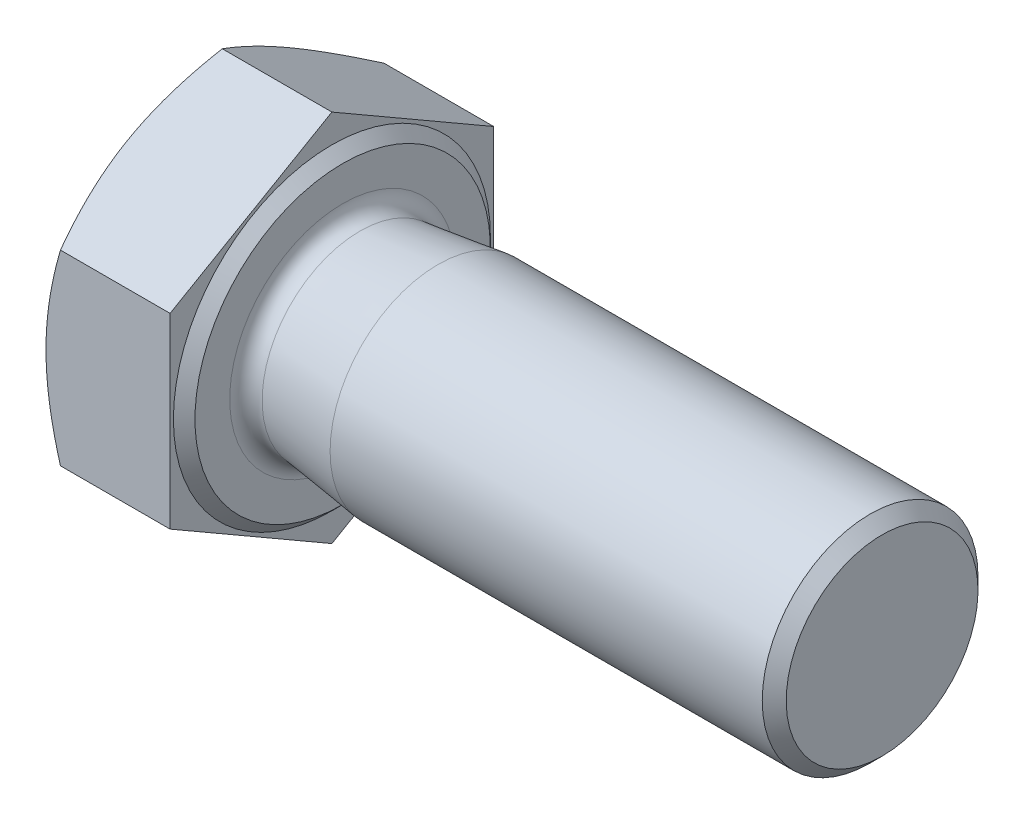
from build123d import *

# Parameters (mm, degrees)
EXTRUDE_1_DEPTH     = 7.5
SKETCH_4_R          = 20.03
SKETCH_4_R_2        = 9
CUT_EXTRUDE_1_DEPTH = 0.9375
CUT_EXTRUDE_1_DRAFT = -60
CHAMFER_1_SIZE      = 0.666666667


with BuildPart() as part:
    # 草图3 → 凸台-拉伸1 (new body)
    with BuildSketch(Plane(origin=(0, 0, 0), x_dir=(0, 0, -1), z_dir=(1, 0, 0))):
        Polygon((9, 5.196152423), (0, 10.392304845), (-9, 5.196152423), (-9, -5.196152423), (0, -10.392304845), (9, -5.196152423), align=None)
    extrude(amount=EXTRUDE_1_DEPTH)


with BuildPart() as cut_extrude_1_tool:
    # 草图4 → 切除-拉伸1 (with draft: the straight prism first)
    with BuildSketch(Plane.ZY):
        Circle(SKETCH_4_R)
        Circle(SKETCH_4_R_2, mode=Mode.SUBTRACT)
    extrude(amount=-CUT_EXTRUDE_1_DEPTH)
    # 切除-拉伸1: the draft: its side faces are tilted about the plane it starts from
    cut_extrude_1_sides = [cut_extrude_1_tool.faces().sort_by_distance(p)[0] for p in [
        (0.46875, 0, -20.03),
        (0.46875, 0, -9),
    ]]
    draft(cut_extrude_1_sides, Plane.ZY, CUT_EXTRUDE_1_DRAFT)


with BuildPart() as part_1:
    add(part.part)

    # 切除-拉伸1: cut by cut_extrude_1_tool
    add(cut_extrude_1_tool.part, mode=Mode.SUBTRACT)

    # 草图6 → 旋转2 (revolve)
    with BuildSketch(Plane.XY, mode=Mode.PRIVATE) as revolve_2_sk:
        with BuildLine():
            Line((12.8, 6), (37.5, 6))
            Line((37.5, 6), (37.5, 0))
            Line((37.5, 0), (7.5, 0))
            Line((7.5, 0), (7.5, 6.2816875))
            ThreePointArc((7.5, 6.2816875), (7.788817563, 5.643272061), (8.458998289, 5.438705073))
            Line((8.458998289, 5.438705073), (12.8, 6))
        make_face()
    revolve(revolve_2_sk.sketch.rotate(Axis((7.5, 0, 0), (1, 0, 0)), 180), axis=Axis((7.5, 0, 0), (1, 0, 0)))

    # 倒角1
    chamfer_1_edges = [part_1.edges().sort_by_distance(p)[0] for p in [
        (37.5, 6, 0),
    ]]
    chamfer(chamfer_1_edges, length=CHAMFER_1_SIZE)

    # 草图8 → 切除-旋转2 (revolve, cut)
    with BuildSketch(Plane.XY, mode=Mode.PRIVATE) as cut_revolve_2_sk:
        Polygon((7.5, 8.215), (6.9, 8.815), (6.9, 20.03), (7.5, 20.03), align=None)
    revolve(cut_revolve_2_sk.sketch.rotate(Axis((0, 0, 0), (1, 0, 0)), 180), axis=Axis((0, 0, 0), (1, 0, 0)), mode=Mode.SUBTRACT)


solid = part_1.part
